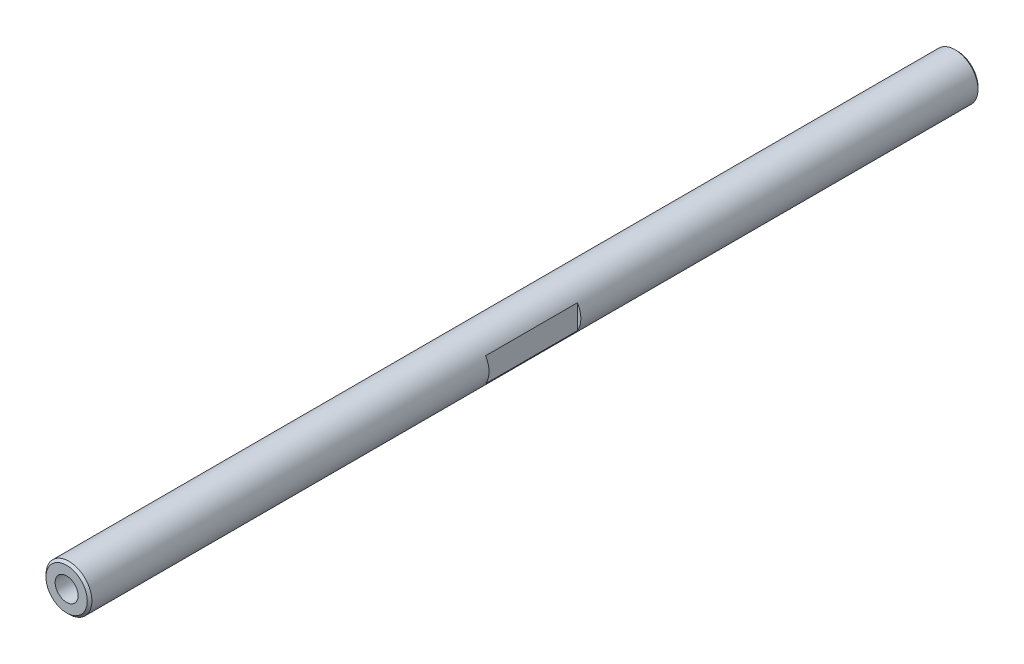
from build123d import *

# Parameters (mm, degrees)
SKETCH_1_R             = 5
EXTRUDE_1_DEPTH        = 97
CUT_EXTRUDE_1_DEPTH    = 10
HOLE_WIZARD_M6_1_D     = 5
HOLE_WIZARD_M6_1_DEPTH = 15
HOLE_WIZARD_M6_1_TIP   = 1.502151548
HOLE_WIZARD_M6_2_D     = 5
HOLE_WIZARD_M6_2_DEPTH = 15
HOLE_WIZARD_M6_2_TIP   = 1.502151548
CHAMFER_1_SIZE         = 0.5


with BuildPart() as part:
    # 草图1 → 凸台-拉伸1 (new, symmetric)
    with BuildSketch(Plane.XY):
        with Locations(Location((0, 0, 0), (0, 0, 180))):
            Circle(SKETCH_1_R)
    extrude(amount=EXTRUDE_1_DEPTH, both=True)

    # 草图2 → 切除-拉伸1 (cut, symmetric)
    with BuildSketch(Plane.XY):
        with BuildLine():
            Line((-4.25, 2.633913438), (-4.25, -2.633913438))
            ThreePointArc((-4.25, -2.633913438), (-5, 0), (-4.25, 2.633913438))
        make_face()
        with BuildLine():
            Line((4.25, 2.633913438), (4.25, -2.633913438))
            ThreePointArc((4.25, -2.633913438), (5, 0), (4.25, 2.633913438))
        make_face()
    extrude(amount=CUT_EXTRUDE_1_DEPTH, both=True, mode=Mode.SUBTRACT)

    # M6 螺纹孔1
    with Locations(Plane.XY.offset(97)):
        with Locations((0, 0)):
            Hole(HOLE_WIZARD_M6_1_D / 2, depth=HOLE_WIZARD_M6_1_DEPTH)
            with Locations((0, 0, -(HOLE_WIZARD_M6_1_DEPTH + HOLE_WIZARD_M6_1_TIP / 2))):  # 118° drill point
                Cone(0, HOLE_WIZARD_M6_1_D / 2, HOLE_WIZARD_M6_1_TIP, mode=Mode.SUBTRACT)

    # M6 螺纹孔2
    with Locations(Plane(origin=(0, 0, -97), x_dir=(-1, 0, 0), z_dir=(0, 0, -1))):
        with Locations((0, 0)):
            Hole(HOLE_WIZARD_M6_2_D / 2, depth=HOLE_WIZARD_M6_2_DEPTH)
            with Locations((0, 0, -(HOLE_WIZARD_M6_2_DEPTH + HOLE_WIZARD_M6_2_TIP / 2))):  # 118° drill point
                Cone(0, HOLE_WIZARD_M6_2_D / 2, HOLE_WIZARD_M6_2_TIP, mode=Mode.SUBTRACT)

    # 倒角1
    chamfer_1_edges = [part.edges().sort_by_distance(p)[0] for p in [
        (5, 0, -97),
        (5, 0, 97),
    ]]
    chamfer(chamfer_1_edges, length=CHAMFER_1_SIZE)


solid = part.part
